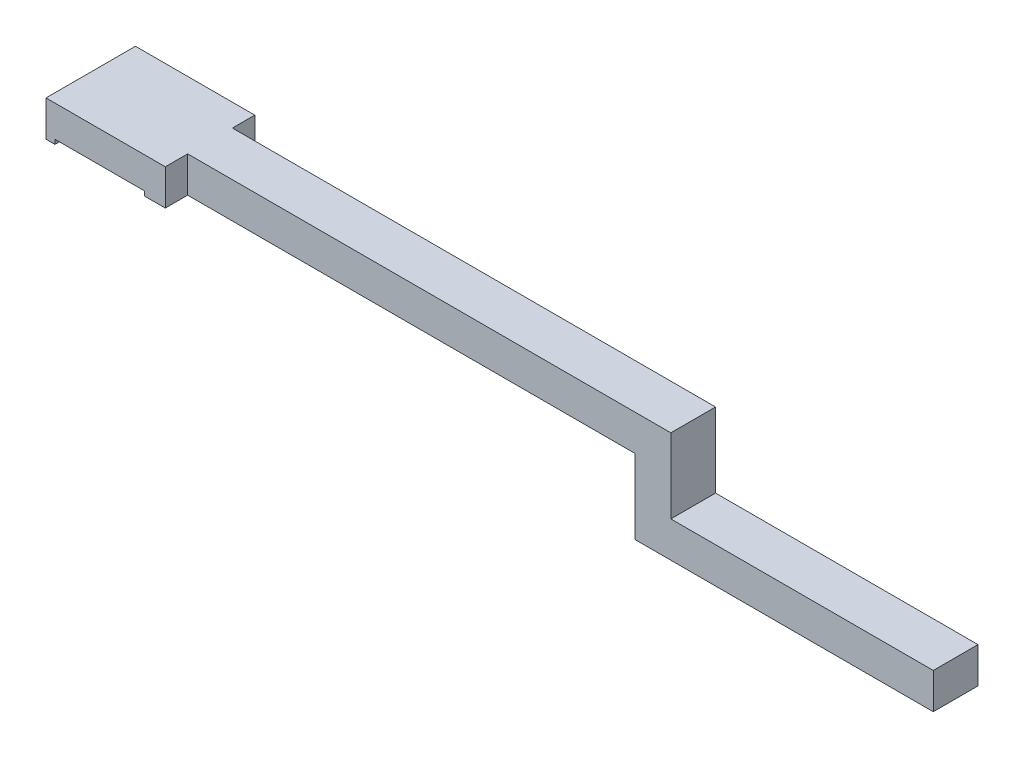
SolidWorks part; units mm, degrees
ref_plane "前视基准面" through (0, 0, 0) normal (0, 0, 1) x (1, 0, 0)
ref_plane "上视基准面" through (0, 0, 0) normal (0, 1, 0) x (1, 0, 0)
ref_plane "右视基准面" through (0, 0, 0) normal (1, 0, 0) x (0, 0, -1)
sketch "草图6" plane through (0, 0, 0) normal (0, 0, 1) x (1, 0, 0)
  line L0 (0, 0) -> (162, 0)
  line L1 (162, 0) -> (162, -25)
  line L2 (162, -25) -> (250, -25)
  line L3 (250, -25) -> (250, -37)
  line L4 (250, -37) -> (150, -37)
  line L5 (150, -37) -> (150, -12)
  line L6 (150, -12) -> (0, -12)
  line L7 (0, -12) -> (0, 0)
  dimension "D1" = 12
  dimension "D2" = 150
  dimension "D3" = 12
  dimension "D4" = 12
  dimension "D5" = 100
  dimension "D6" = 25
extrude "凸台-拉伸5" add sketch "草图6" along normal mid plane 15
sketch "草图7" plane through (0, 0, 0) normal (0, 1, 0) x (1, 0, 0)
  line L0 (0, -7.5) -> (0, 7.5) construction
  line L1 (0, -15) -> (-40, -15)
  line L2 (0, -15) -> (0, 15)
  line L3 (0, 15) -> (-40, 15)
  line L4 (-40, -15) -> (-40, 15)
  line L5 (0, -15) -> (-40, 15) construction
  line L6 (0, 15) -> (-40, -15) construction
  point P0 (-20, 0)
  dimension "D1" = 30
  dimension "D2" = 40
extrude "凸台-拉伸6" add sketch "草图7" against normal up to surface (12 mm away) up to face at (75, -12, 0)
sketch "草图8" plane through (0, -12, 0) normal (0, 1, 0) x (1, 0, 0)
  line L0 (0, 15) -> (-40, 15) construction
  line L1 (-37, 15) -> (-7, 15)
  line L2 (-37, 15) -> (-37, -15)
  line L3 (-37, -15) -> (-7, -15)
  line L4 (-7, 15) -> (-7, -15)
  line L5 (-40, -15) -> (0, -15) construction
  line L6 (-40, 15) -> (-40, -15) construction
  dimension "D1" = 30
  dimension "D2" = 3
extrude "切除-拉伸1" cut sketch "草图8" along normal blind 1.5
